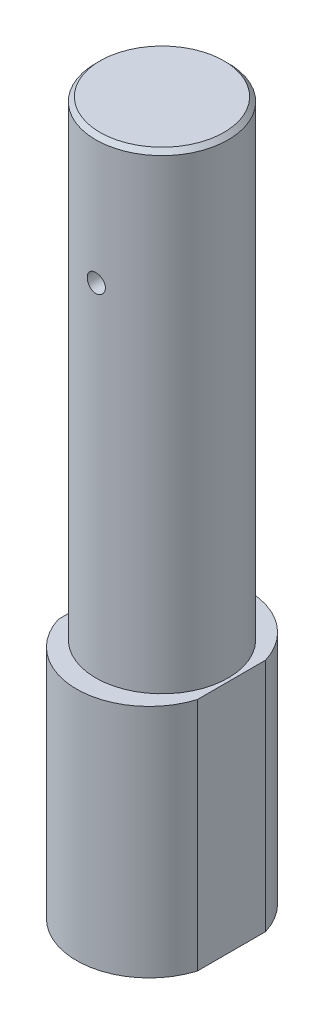
from build123d import *

# Parameters (mm, degrees)
EXTRUDE_1_DEPTH         = 110
SKETCH_2_R              = 31
EXTRUDE_2_DEPTH         = 220
HOLE_WIZARD_M10_1_D     = 8.5
HOLE_WIZARD_M10_1_DEPTH = 27.5
HOLE_WIZARD_M10_1_TIP   = 2.553657631
CHAMFER_1_SIZE          = 2


with BuildPart() as part:
    # 草图1 → 凸台-拉伸1 (new body)
    with BuildSketch(Plane(origin=(0, 0, 0), x_dir=(1, 0, 0), z_dir=(0, 1, 0))):
        with BuildLine():
            Line((32.5, -15.987492178), (32.5, 15.987492178))
            ThreePointArc((32.5, 15.987492178), (0, 40), (-32.5, 15.987492178))
            Line((-32.5, 15.987492178), (-32.5, -15.987492178))
            ThreePointArc((-32.5, -15.987492178), (0, -40), (32.5, -15.987492178))
        make_face()
    extrude(amount=EXTRUDE_1_DEPTH)

    # 草图2 → 凸台-拉伸2 (add)
    with BuildSketch(Plane(origin=(0, 110, 0), x_dir=(1, 0, 0), z_dir=(0, 1, 0))):
        with Locations(Location((0, 0, 0), (0, 0, 270))):
            Circle(SKETCH_2_R)
    extrude(amount=EXTRUDE_2_DEPTH)

    # M10 螺纹孔1
    with Locations(Plane.XY.offset(31)):
        with Locations((0, 270)):
            Hole(HOLE_WIZARD_M10_1_D / 2, depth=HOLE_WIZARD_M10_1_DEPTH)
            with Locations((0, 0, -(HOLE_WIZARD_M10_1_DEPTH + HOLE_WIZARD_M10_1_TIP / 2))):  # 118° drill point
                Cone(0, HOLE_WIZARD_M10_1_D / 2, HOLE_WIZARD_M10_1_TIP, mode=Mode.SUBTRACT)

    # 倒角1
    chamfer_1_edges = [part.edges().sort_by_distance(p)[0] for p in [
        (0, 330, -31),
    ]]
    chamfer(chamfer_1_edges, length=CHAMFER_1_SIZE)

    # 草图5 → 切除-旋转1 (revolve, cut)
    with BuildSketch(Plane.XY):
        with BuildLine():
            Line((0, 23), (0, -33))
            ThreePointArc((0, -33), (28, -5), (0, 23))
        make_face()
    revolve(axis=Axis((0, 23, 0), (0, -1, 0)), mode=Mode.SUBTRACT)


solid = part.part
